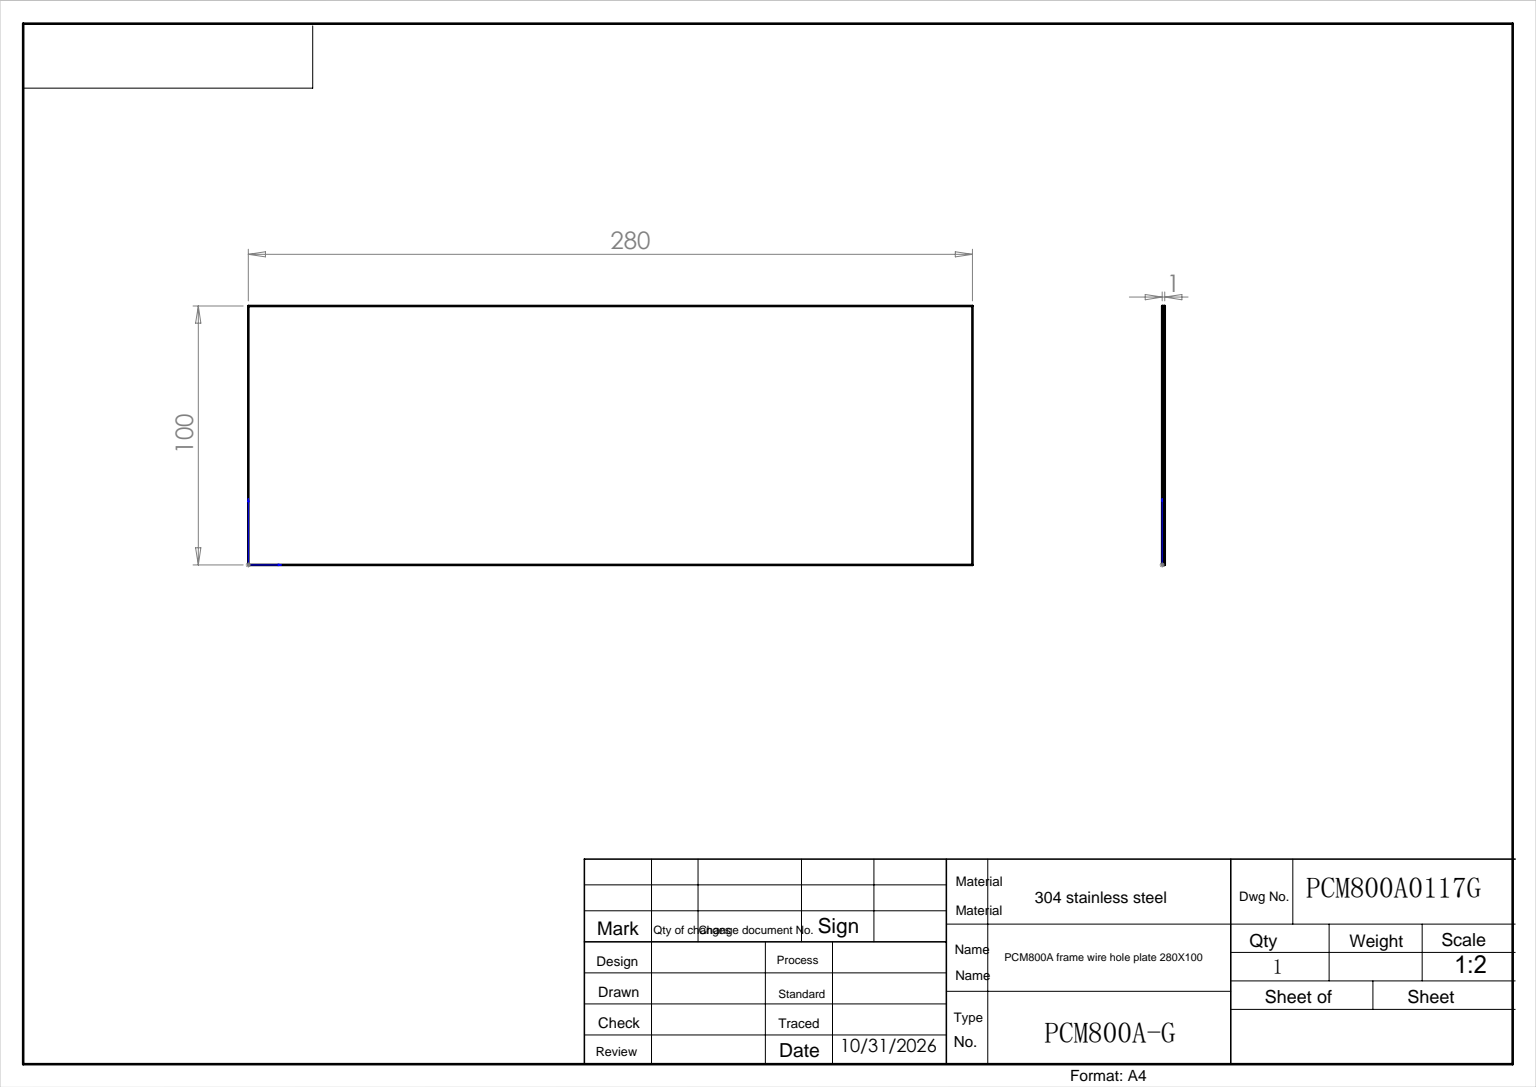
from build123d import *

# Parameters (mm, degrees)
SKETCH_1_W      = 280
SKETCH_1_H      = 100
EXTRUDE_1_DEPTH = 1


with BuildPart() as part:
    # 草图1 → 凸台-拉伸1 (new body)
    with BuildSketch(Plane.XY):
        with Locations((140, 50)):
            Rectangle(SKETCH_1_W, SKETCH_1_H)
    extrude(amount=EXTRUDE_1_DEPTH)


solid = part.part
